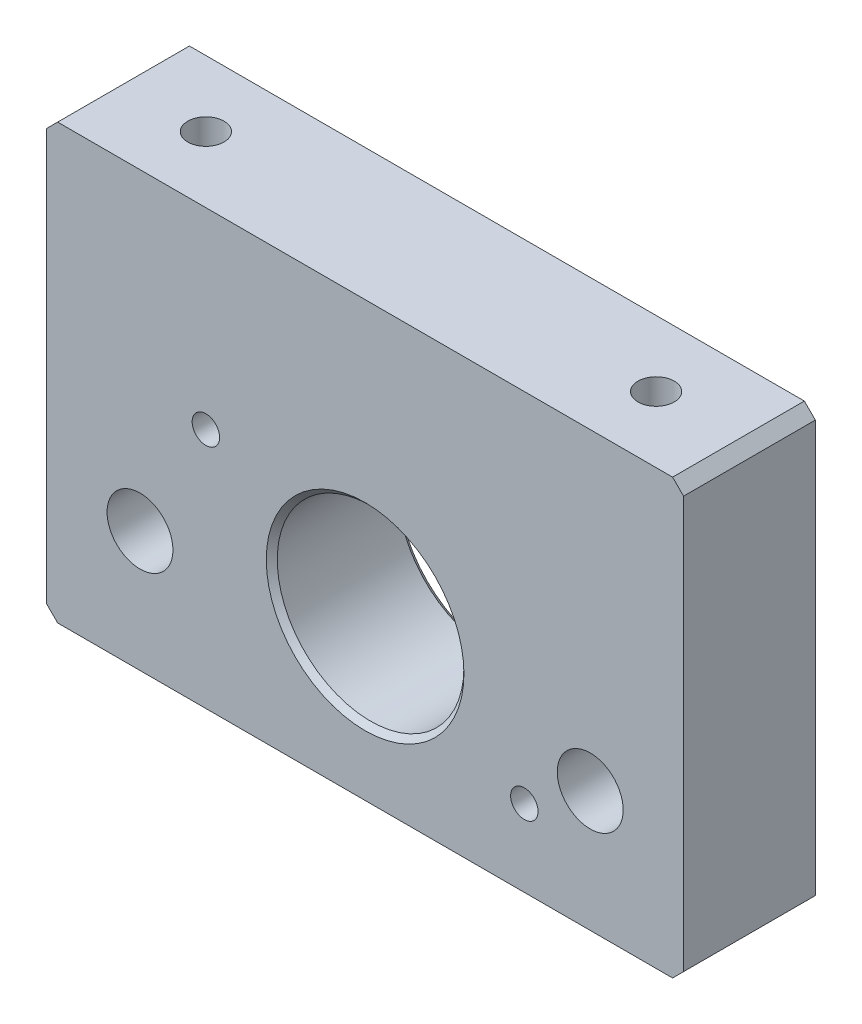
from build123d import *

# Parameters (mm, degrees)
SKETCH1_W                  = 58
SKETCH1_H                  = 39.5
SKETCH1_R                  = 8.5
SKETCH1_R_2                = 3
BOSS_EXTRUDE1_DEPTH        = 6
M3_TAPPED_HOLE1_D          = 2.5
M4_TAPPED_HOLE1_AT_2_COUNT = 2
M4_TAPPED_HOLE1_AT_2_PITCH = 41
CHAMFER1_SIZE              = 1
CHAMFER2_SIZE              = 0.5


with BuildPart() as part:
    # Sketch1 → Boss-Extrude1 (new, symmetric)
    with BuildSketch(Plane.XY):
        Rectangle(SKETCH1_W, SKETCH1_H)
        with Locations((0, -5.25)):
            Circle(SKETCH1_R, mode=Mode.SUBTRACT)
        with Locations((-20.5, -8.75)):
            Circle(SKETCH1_R_2, mode=Mode.SUBTRACT)
        with Locations((20.5, -8.75)):
            Circle(SKETCH1_R_2, mode=Mode.SUBTRACT)
    extrude(amount=BOSS_EXTRUDE1_DEPTH, both=True)

    # M3 Tapped Hole1 (through all)
    with Locations(Plane.XY.offset(6)):
        with Locations((-14.5, 2.25), (14.5, -12.75)):
            Hole(M3_TAPPED_HOLE1_D / 2)

    # Sketch4 → M4 Tapped Hole1 (revolve, cut)
    with BuildSketch(Plane(origin=(-20.5, -19.75, 0), x_dir=(0, 0, -1), z_dir=(1, 0, 0))):
        Polygon((0, 0), (0, 11.091420021), (1.65, 10.1), (1.65, 0), align=None)
    m4_tapped_hole1 = revolve(axis=Axis((-20.5, -26.1, 0), (0, 1, 0)), mode=Mode.SUBTRACT)

    # M4 Tapped Hole1 at 2: M4 Tapped Hole1 ×2
    with Locations(*[(i * M4_TAPPED_HOLE1_AT_2_PITCH, 0, 0) for i in range(1, M4_TAPPED_HOLE1_AT_2_COUNT)]):
        add(m4_tapped_hole1, mode=Mode.SUBTRACT)

    # Mirror1: M4 Tapped Hole1 across plane
    add(m4_tapped_hole1.mirror(Plane.ZX), mode=Mode.SUBTRACT)

    # Mirror1 copy 1 sketch → Mirror1 copy 1 (revolve, cut)
    with BuildSketch(Plane(origin=(20.5, 19.75, 0), x_dir=(0, 0, -1), z_dir=(1, 0, 0))):
        Polygon((0, 0), (0, -11.091420021), (1.65, -10.1), (1.65, 0), align=None)
    revolve(axis=Axis((20.5, 26.1, 0), (0, 1, 0)), mode=Mode.SUBTRACT)

    # Chamfer1
    chamfer1_edges = [part.edges().sort_by_distance(p)[0] for p in [
        (29, -19.75, 0),
        (-29, -19.75, 0),
        (-29, 19.75, 0),
        (29, 19.75, 0),
    ]]
    chamfer(chamfer1_edges, length=CHAMFER1_SIZE)

    # Chamfer2
    chamfer2_edges = [part.edges().sort_by_distance(p)[0] for p in [
        (-8.5, -5.25, -6),
        (-8.5, -5.25, 6),
    ]]
    chamfer(chamfer2_edges, length=CHAMFER2_SIZE)


solid = part.part
